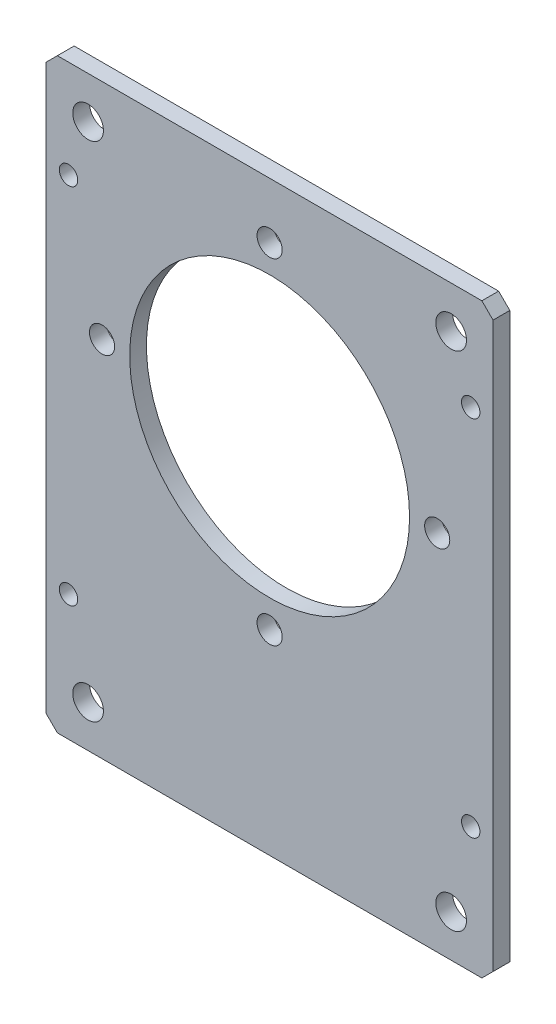
from build123d import *

# Parameters (mm, degrees)
SKETCH1_W                  = 80
SKETCH1_H                  = 105
BOSS_EXTRUDE1_DEPTH        = 3
SKETCH2_R                  = 2.75
SKETCH2_R_2                = 25.05
CUT_EXTRUDE1_DEPTH         = 133.037873355
F_4_5_4_5_DIAMETER_HOLE1_D = 4.5
CHAMFER1_SIZE              = 2
M4_TAPPED_HOLE1_D          = 3.3
M4_TAPPED_HOLE1_DEPTH      = 10.1
M4_TAPPED_HOLE1_TIP        = 0.991420021


with BuildPart() as part:
    # Sketch1 → Boss-Extrude1 (new body)
    with BuildSketch(Plane.XY):
        with Locations((40, 52.5)):
            Rectangle(SKETCH1_W, SKETCH1_H)
    extrude(amount=BOSS_EXTRUDE1_DEPTH)

    # Sketch2 → Cut-Extrude1 (cut, through all)
    with BuildSketch(Plane.XY.offset(3)):
        with Locations((7.5, 97.5)):
            Circle(SKETCH2_R)
        with Locations((72.5, 97.5)):
            Circle(SKETCH2_R)
        with Locations((72.5, 7.5)):
            Circle(SKETCH2_R)
        with Locations((7.5, 7.5)):
            Circle(SKETCH2_R)
        with Locations((40, 65)):
            Circle(SKETCH2_R_2)
    extrude(amount=-CUT_EXTRUDE1_DEPTH, mode=Mode.SUBTRACT)

    # Ø4.5 (4.5) Diameter Hole1 (through all)
    with Locations(Plane.XY.offset(3)):
        with Locations((40, 95), (10, 65), (70, 65), (40, 35)):
            Hole(F_4_5_4_5_DIAMETER_HOLE1_D / 2)

    # Chamfer1
    chamfer1_edges = [part.edges().sort_by_distance(p)[0] for p in [
        (0, 105, 1.5),
        (80, 105, 1.5),
        (80, 0, 1.5),
        (0, 0, 1.5),
    ]]
    chamfer(chamfer1_edges, length=CHAMFER1_SIZE)

    # M4 Tapped Hole1
    with Locations(Plane.XY.offset(3)):
        with Locations((4, 87.5), (76, 87.5), (76, 22.5), (4, 22.5), (40, 65)):
            Hole(M4_TAPPED_HOLE1_D / 2, depth=M4_TAPPED_HOLE1_DEPTH)
            with Locations((0, 0, -(M4_TAPPED_HOLE1_DEPTH + M4_TAPPED_HOLE1_TIP / 2))):  # 118° drill point
                Cone(0, M4_TAPPED_HOLE1_D / 2, M4_TAPPED_HOLE1_TIP, mode=Mode.SUBTRACT)


solid = part.part
